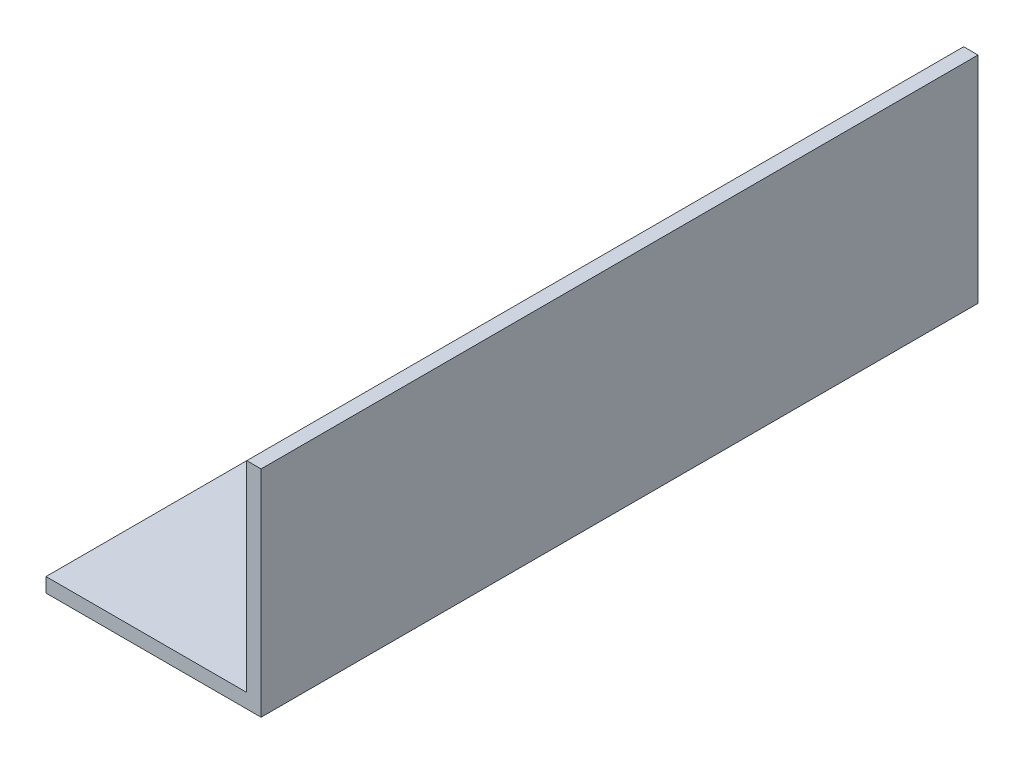
from build123d import *

# Parameters (mm, degrees)
EXTRUDE_2_DEPTH = 100


with BuildPart() as part:
    # 草图1 → 凸台-拉伸2 (new body)
    with BuildSketch(Plane.XY):
        Polygon((0, 0), (30, 0), (30, 30), (28, 30), (28, 2), (0, 2), align=None)
    extrude(amount=EXTRUDE_2_DEPTH)


solid = part.part
